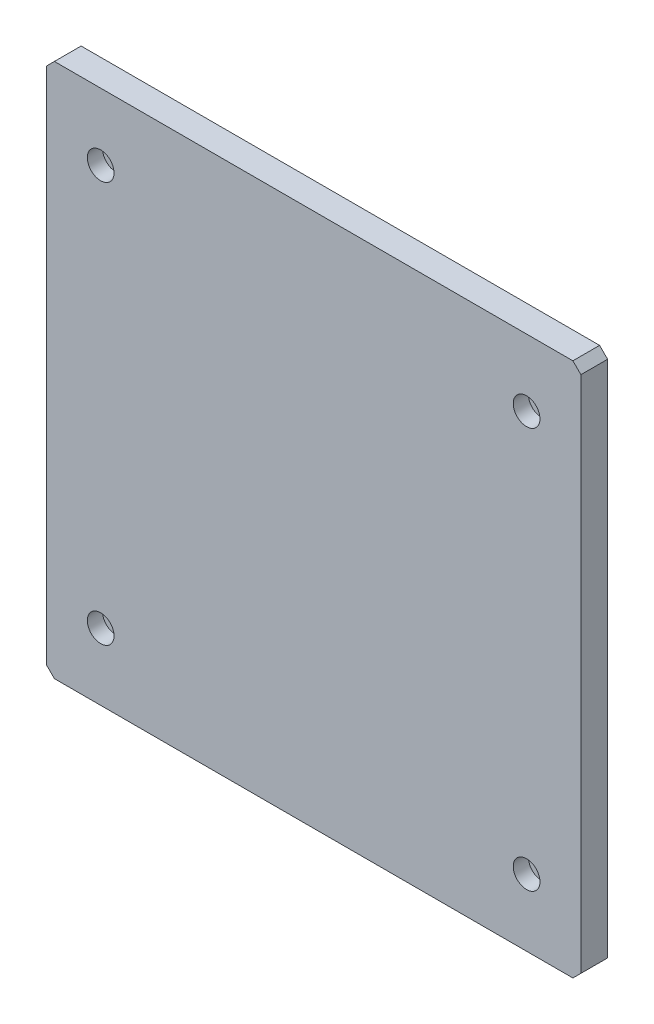
from build123d import *

# Parameters (mm, degrees)
SKETCH1_W                                            = 200
SKETCH1_H                                            = 200
BOSS_EXTRUDE1_DEPTH                                  = 10
CBORE_FOR_M5_HEXAGON_SOCKET_HEAD_CAP_SCR_D           = 5.5
CBORE_FOR_M5_HEXAGON_SOCKET_HEAD_CAP_SCR_DEPTH       = 36.9
CBORE_FOR_M5_HEXAGON_SOCKET_HEAD_CAP_SCR_CBORE_D     = 10
CBORE_FOR_M5_HEXAGON_SOCKET_HEAD_CAP_SCR_CBORE_DEPTH = 5.7
CBORE_FOR_M5_HEXAGON_SOCKET_HEAD_CAP_SCR_TIP         = 1.652366702
CHAMFER1_SIZE                                        = 3


with BuildPart() as part:
    # Sketch1 → Boss-Extrude1 (new body)
    with BuildSketch(Plane.XY):
        Rectangle(SKETCH1_W, SKETCH1_H)
    extrude(amount=BOSS_EXTRUDE1_DEPTH)

    # CBORE for M5 Hexagon socket head cap screws1
    with Locations(Plane.XY.offset(10)):
        with Locations((-79.680151025, 75), (79.680151025, 75), (79.680151025, -75), (-79.680151025, -75)):
            CounterBoreHole(CBORE_FOR_M5_HEXAGON_SOCKET_HEAD_CAP_SCR_D / 2, CBORE_FOR_M5_HEXAGON_SOCKET_HEAD_CAP_SCR_CBORE_D / 2, CBORE_FOR_M5_HEXAGON_SOCKET_HEAD_CAP_SCR_CBORE_DEPTH, depth=CBORE_FOR_M5_HEXAGON_SOCKET_HEAD_CAP_SCR_DEPTH)
            with Locations((0, 0, -(CBORE_FOR_M5_HEXAGON_SOCKET_HEAD_CAP_SCR_DEPTH + CBORE_FOR_M5_HEXAGON_SOCKET_HEAD_CAP_SCR_TIP / 2))):  # 118° drill point
                Cone(0, CBORE_FOR_M5_HEXAGON_SOCKET_HEAD_CAP_SCR_D / 2, CBORE_FOR_M5_HEXAGON_SOCKET_HEAD_CAP_SCR_TIP, mode=Mode.SUBTRACT)

    # Chamfer1
    chamfer1_edges = [part.edges().sort_by_distance(p)[0] for p in [
        (100, -100, 5),
        (-100, -100, 5),
        (-100, 100, 5),
        (100, 100, 5),
    ]]
    chamfer(chamfer1_edges, length=CHAMFER1_SIZE)


solid = part.part
